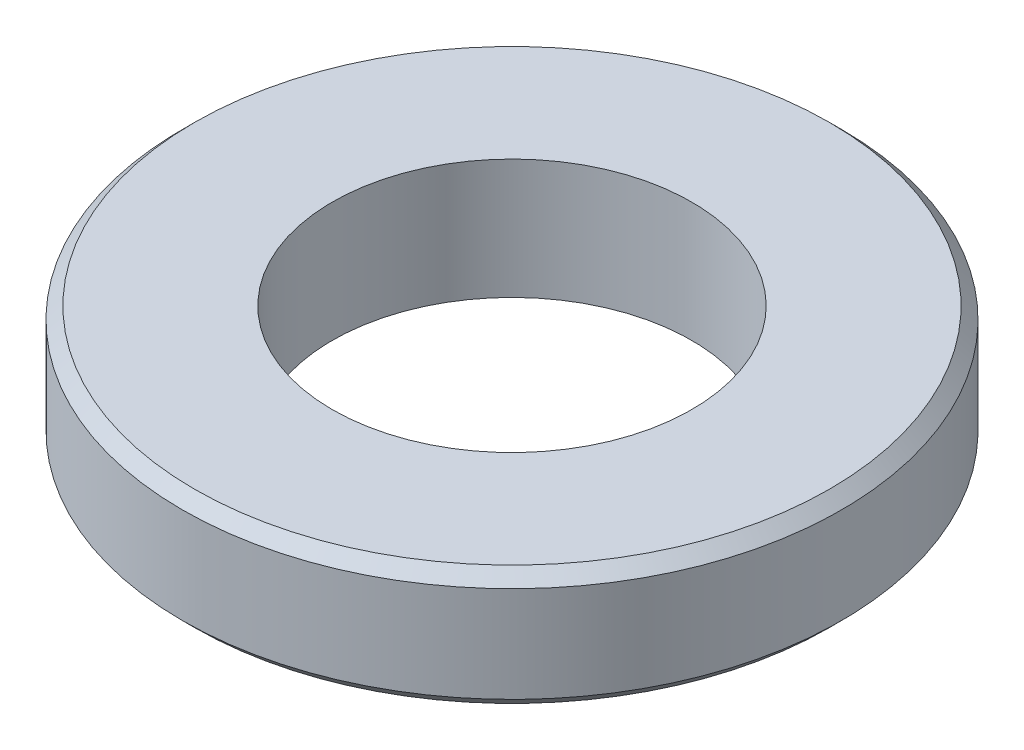
from build123d import *

# Parameters (mm, degrees)
SKETCH1_R           = 2.75
SKETCH1_R_2         = 1.5
BOSS_EXTRUDE1_DEPTH = 1
CHAMFER1_SIZE       = 0.1


with BuildPart() as part:
    # Sketch1 → Boss-Extrude1 (new body)
    with BuildSketch(Plane(origin=(0, 0, 0), x_dir=(1, 0, 0), z_dir=(0, 1, 0))):
        with Locations(Location((0, 0, 0), (0, 0, 270))):
            Circle(SKETCH1_R)
        with Locations(Location((0, 0, 0), (0, 0, 270))):
            Circle(SKETCH1_R_2, mode=Mode.SUBTRACT)
    extrude(amount=BOSS_EXTRUDE1_DEPTH)

    # Chamfer1
    chamfer1_edges = [part.edges().sort_by_distance(p)[0] for p in [
        (0, 0, -2.75),
        (0, 1, -2.75),
    ]]
    chamfer(chamfer1_edges, length=CHAMFER1_SIZE)


solid = part.part
